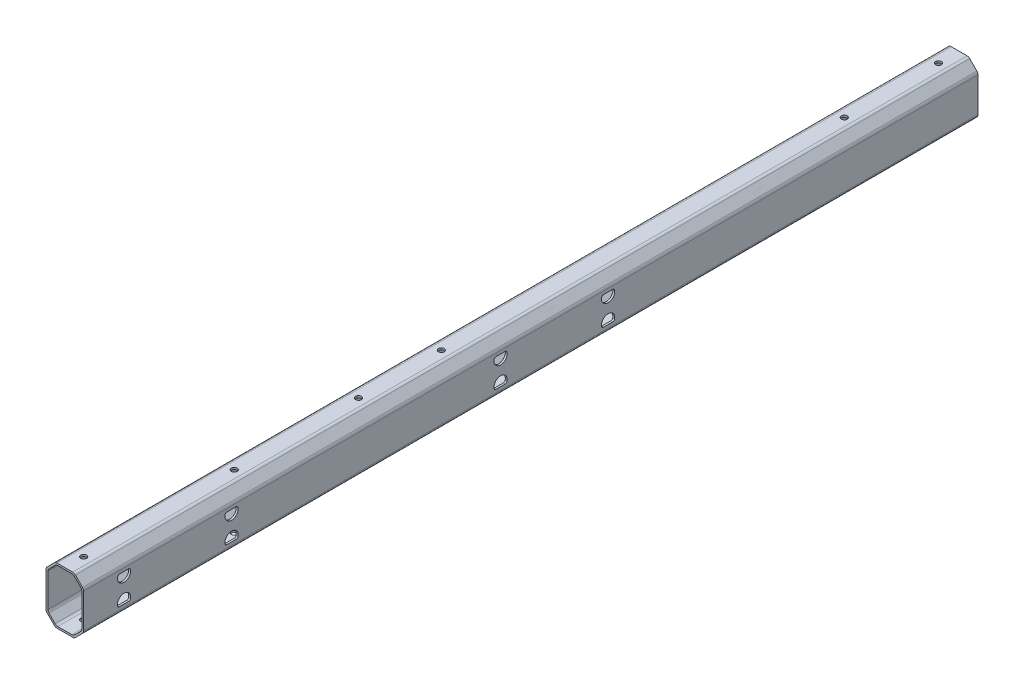
SolidWorks part; units mm, degrees
material "Thornel Mat VMA"
ref_plane "前视基准面" through (0, 0, 0) normal (0, 0, 1) x (1, 0, 0)
ref_plane "上视基准面" through (0, 0, 0) normal (0, 1, 0) x (1, 0, 0)
ref_plane "右视基准面" through (0, 0, 0) normal (1, 0, 0) x (0, 0, -1)
other "Configuration Table"
sketch "草图1" plane through (0, 0, 0) normal (0, 0, 1) x (1, 0, 0)
  line L0 (-5, 15) -> (5, 15)
  line L1 (-10, 15) -> (10, 15) construction
  line L2 (-10, 15) -> (-10, -15) construction
  line L3 (-10, -15) -> (10, -15) construction
  line L4 (10, 15) -> (10, -15) construction
  line L5 (-10, 15) -> (10, -15) construction
  line L6 (-10, -15) -> (10, 15) construction
  line L7 (5, 15) -> (10, 10)
  line L8 (10, 10) -> (10, -10)
  line L9 (10, -10) -> (5, -15)
  line L10 (5, -15) -> (-5, -15)
  line L11 (-5, -15) -> (-10, -10)
  line L12 (-10, -10) -> (-10, 10)
  line L13 (-10, 10) -> (-5, 15)
  line L14 (0, 0) -> (10, 0) construction
  line L15 (0, 0) -> (0, 15) construction
  line L16 (-9, 9.5858) -> (-4.5858, 14)
  line L17 (-4.5858, 14) -> (4.5858, 14)
  line L18 (4.5858, 14) -> (9, 9.5858)
  line L19 (9, 9.5858) -> (9, -9.5858)
  line L20 (9, -9.5858) -> (4.5858, -14)
  line L21 (4.5858, -14) -> (-4.5858, -14)
  line L22 (-4.5858, -14) -> (-9, -9.5858)
  line L23 (-9, -9.5858) -> (-9, 9.5858)
  point P0 (0, 0)
  dimension "D1" = 20
  dimension "D2" = 30
  dimension "D3" = 45
  dimension "D4" = 1
  dimension "D5" = 10
extrude "凸台-拉伸1" add sketch "草图1" along normal blind 475
fillet "圆角1" radius 2 16 edges at (-5, -15, 237.5) (-10, -10, 237.5) (5, -15, 237.5) (10, -10, 237.5) (10, 10, 237.5) (5, 15, 237.5) (-5, 15, 237.5) (-10, 10, 237.5) (-9, -9.5858, 237.5) (-4.5858, -14, 237.5) (4.5858, -14, 237.5) (9, -9.5858, 237.5) (9, 9.5858, 237.5) (4.5858, 14, 237.5) (-4.5858, 14, 237.5) (-9, 9.5858, 237.5)
sketch "草图2" plane through (0, 15, 0) normal (0, 1, 0) x (1, 0, 0)
  line L1 (10, 0) -> (10, -475) construction
  line L2 (4.1716, 0) -> (-4.1716, 0) construction
  circle A0 centre (0, -11) radius 1.55
  circle A1 centre (0, -61) radius 1.55
  circle A2 centre (0, -425) radius 9 construction
  circle A3 centre (0, -385) radius 1.55
  circle A4 centre (0, -465) radius 1.55
  circle A5 centre (0, -319) radius 1.55
  circle A6 centre (0, -275) radius 1.55
  point P17 (0, 0)
  dimension "D1" = 3.1
  dimension "D2" = 11
  dimension "D4" = 50
  dimension "D5" = 425
  dimension "D6" = 18
  dimension "D7" = 3.1
  dimension "D8" = 40
  dimension "D9" = 40
  dimension "D11" = 44
  dimension "D10" = 66
  dimension "D3" = 10
extrude "切除-拉伸1" cut sketch "草图2" against normal through all
sketch "草图3" plane through (-10, 0, 0) normal (-1, 0, 0) x (0, 0, 1)
  line L0 (0, 15) -> (475, 15) construction
  line L1 (396.45, 6) -> (453.55, 6) construction
  line L2 (396.45, 6) -> (396.45, -6) construction
  line L3 (396.45, -6) -> (453.55, -6) construction
  line L4 (453.55, 6) -> (453.55, -6) construction
  line L5 (396.45, 6) -> (453.55, -6) construction
  line L6 (396.45, -6) -> (453.55, 6) construction
  line L8 (196.45, 6) -> (253.55, 6) construction
  line L9 (196.45, 6) -> (196.45, -6) construction
  line L10 (196.45, -6) -> (253.55, -6) construction
  line L11 (253.55, 6) -> (253.55, -6) construction
  line L12 (196.45, 6) -> (253.55, -6) construction
  line L13 (196.45, -6) -> (253.55, 6) construction
  circle A0 centre (396.45, 6) radius 1.05
  circle A1 centre (396.45, -6) radius 1.05
  circle A2 centre (453.55, 6) radius 1.05
  circle A3 centre (453.55, -6) radius 1.05
  circle A4 centre (196.45, 6) radius 1.05
  circle A5 centre (196.45, -6) radius 1.05
  circle A6 centre (253.55, 6) radius 1.05
  circle A7 centre (253.55, -6) radius 1.05
  point P0 (425, 0)
  point P15 (225, 0)
  dimension "D5" = 2.1
  dimension "D6" = 2
  dimension "D1" = 57.1
  dimension "D2" = 12
  dimension "D3" = 15
  dimension "D4" = 425
  dimension "D7" = 200
extrude "切除-拉伸2" cut sketch "草图3" against normal through all both and the other way through all
sketch "草图4" plane through (10, 0, 0) normal (1, 0, 0) x (0, 0, -1)
  line L0 (-458.05, 27.1435) -> (-458.05, -26.8137) construction
  line L1 (-453.55, 6) -> (-396.45, 6) construction
  line L2 (-425, 6) -> (-425, 32.9217) construction
  line L3 (-456.7123, 7.5) -> (-450.3877, 7.5)
  line L4 (-456.7123, -7.5) -> (-450.3877, -7.5)
  line L5 (-393.2877, -7.5) -> (-399.6123, -7.5)
  line L6 (-393.2877, 7.5) -> (-399.6123, 7.5)
  line L7 (-256.7123, 7.5) -> (-250.3877, 7.5)
  line L8 (-256.7123, -7.5) -> (-250.3877, -7.5)
  line L9 (-193.2877, -7.5) -> (-199.6123, -7.5)
  line L10 (-193.2877, 7.5) -> (-199.6123, 7.5)
  line L12 (-253.55, 6) -> (-196.45, 6) construction
  line L13 (-258.05, 27.1435) -> (-258.05, -26.8137) construction
  circle A0 centre (-396.45, 6) radius 1.05 construction
  circle A1 centre (-396.45, -6) radius 1.05 construction
  circle A2 centre (-453.55, -6) radius 1.05 construction
  circle A3 centre (-453.55, 6) radius 1.05 construction
  circle A4 centre (-396.45, 6) radius 1.05 construction
  circle A5 centre (-396.45, -6) radius 1.05 construction
  circle A6 centre (-453.55, -6) radius 1.05 construction
  circle A7 centre (-453.55, 6) radius 1.05 construction
  circle A8 centre (-453.55, 6) radius 3.5
  circle A9 centre (-453.55, -6) radius 3.5
  circle A10 centre (-396.45, -6) radius 3.5
  circle A11 centre (-396.45, 6) radius 3.5
  circle A12 centre (-253.55, 6) radius 3.5
  circle A13 centre (-253.55, -6) radius 3.5
  circle A14 centre (-196.45, -6) radius 3.5
  circle A15 centre (-196.45, 6) radius 3.5
  circle A16 centre (-196.45, 6) radius 1.05 construction
  circle A17 centre (-196.45, -6) radius 1.05 construction
  circle A18 centre (-253.55, -6) radius 1.05 construction
  circle A19 centre (-253.55, 6) radius 1.05 construction
  circle M6 centre (-396.45, -6) radius 1.05
  circle M7 centre (-453.55, 6) radius 1.05
  circle M8 centre (-453.55, -6) radius 1.05
  circle M9 centre (-396.45, 6) radius 1.05
  circle M28 centre (-196.45, 6) radius 1.05
  circle M29 centre (-253.55, -6) radius 1.05
  circle M30 centre (-253.55, 6) radius 1.05
  circle M31 centre (-196.45, -6) radius 1.05
  dimension "D2" = 7
  dimension "D3" = 1.5
  dimension "D1" = 4.5
  dimension "D4" = 1.5
  dimension "D5" = 2
extrude "切除-拉伸3" cut sketch "草图4" against normal up to surface (1 mm away) contours L3 A8 M7 | L4 A9 M8 | A10 L5 M6 | A11 L6 M9 | L7 A12 M30 | L8 A13 M29 | A15 L10 M28 | A14 L9 M31 up to face at (9, 4.95, 196.45)
fillet "圆角2" radius 1 16 edges at (9.5, -7.5, 393.2877) (9.5, -7.5, 399.6123) (9.5, 7.5, 393.2877) (9.5, 7.5, 399.6123) (9.5, -7.5, 450.3877) (9.5, -7.5, 456.7123) (9.5, 7.5, 450.3877) (9.5, 7.5, 456.7123) (9.5, 7.5, 193.2877) (9.5, 7.5, 199.6123) (9.5, -7.5, 199.6123) (9.5, -7.5, 193.2877) (9.5, -7.5, 250.3877) (9.5, -7.5, 256.7123) (9.5, 7.5, 250.3877) (9.5, 7.5, 256.7123)
